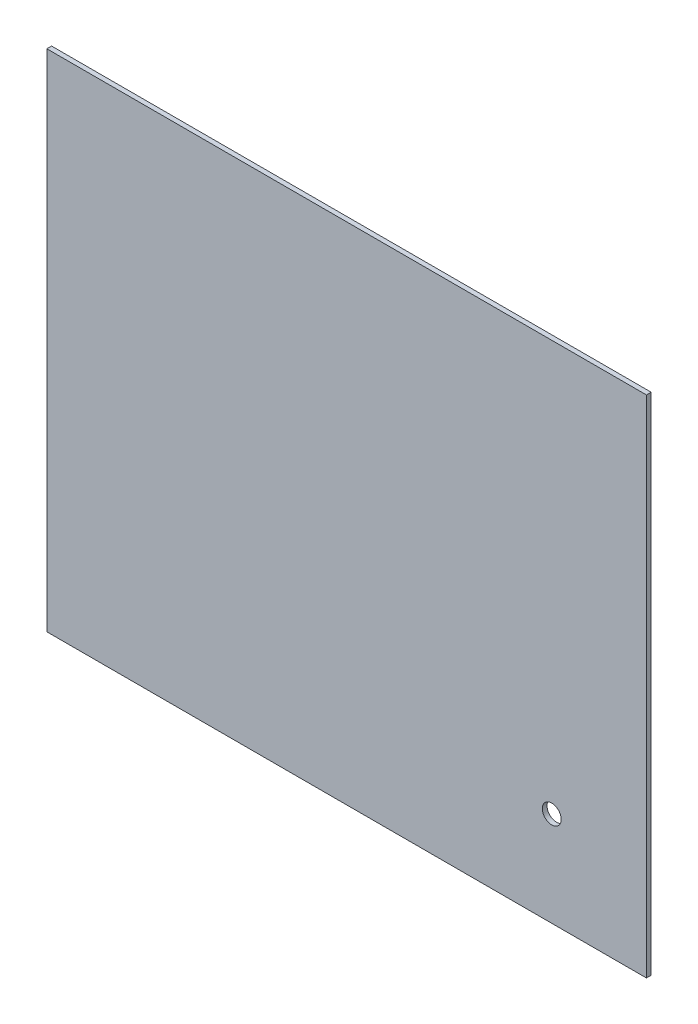
SolidWorks part; units mm, degrees
ref_plane "前视基准面" through (0, 0, 0) normal (0, 0, 1) x (1, 0, 0)
ref_plane "上视基准面" through (0, 0, 0) normal (0, 1, 0) x (1, 0, 0)
ref_plane "右视基准面" through (0, 0, 0) normal (1, 0, 0) x (0, 0, -1)
other "Configuration Table"
sketch "草图1" plane through (0, 0, 0) normal (0, 0, 1) x (1, 0, 0)
  line L0 (-190, -160) -> (190, -160)
  line L1 (190, -160) -> (190, 160)
  line L2 (190, 160) -> (-190, 160)
  line L3 (-190, 160) -> (-190, -160)
  point P0 (0, 0)
  dimension "D1" = 190
  dimension "D2" = 380
  dimension "D3" = 160
  dimension "D4" = 320
extrude "凸台-拉伸1" add sketch "草图1" against normal mid plane 3
sketch "草图2" plane through (0, 0, 0) normal (0, 0, 1) x (1, 0, 0)
  circle A0 centre (130, -100) radius 6
  point P0 (0, 0)
  dimension "D1" = 12
  dimension "D2" = 130
  dimension "D3" = 100
extrude "切除-拉伸1" cut sketch "草图2" against normal mid plane 23
